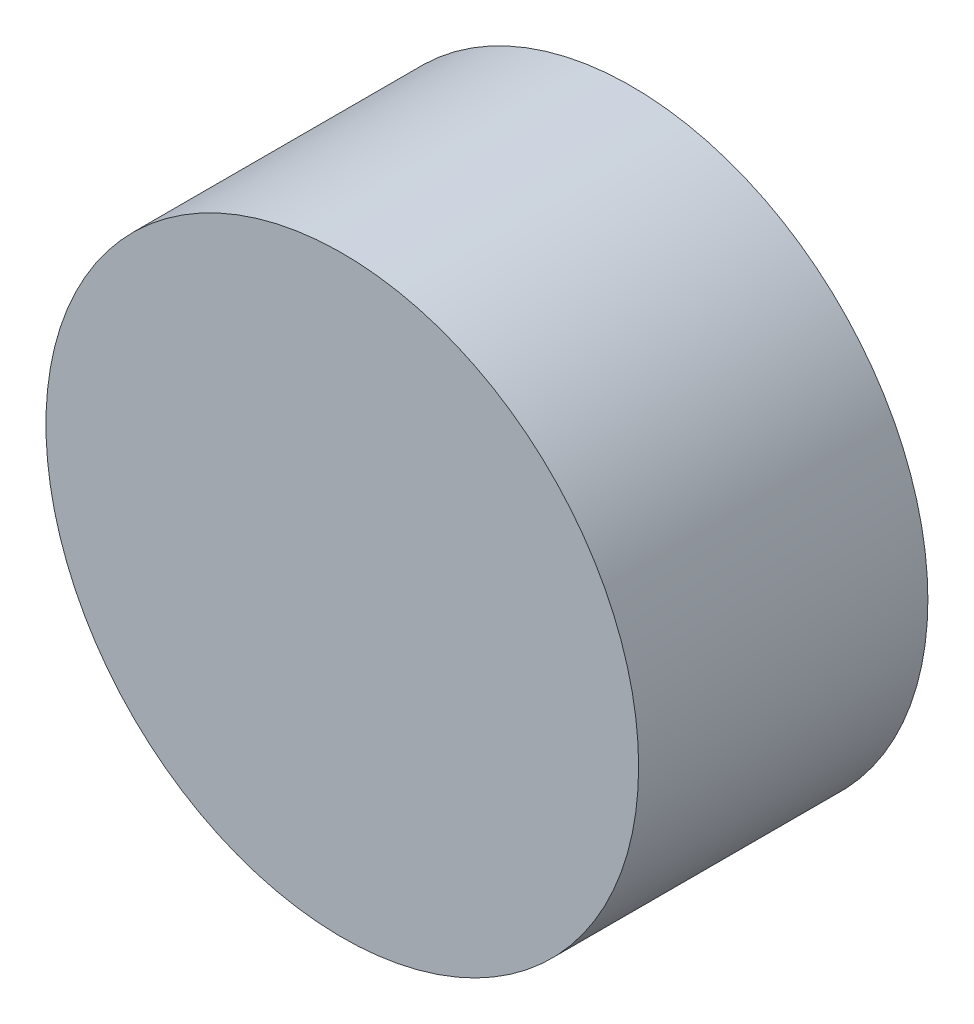
SolidWorks part; units mm, degrees
ref_plane "Front Plane" through (0, 0, 0) normal (0, 0, 1) x (1, 0, 0)
ref_plane "Top Plane" through (0, 0, 0) normal (0, 1, 0) x (1, 0, 0)
ref_plane "Right Plane" through (0, 0, 0) normal (1, 0, 0) x (0, 0, -1)
sketch "Sketch1" plane through (0, 0, 0) normal (0, 0, 1) x (1, 0, 0)
  circle A0 centre (-138.8634, 112.983) radius 10.2452
extrude "Boss-Extrude1" add sketch "Sketch1" along normal blind 10
